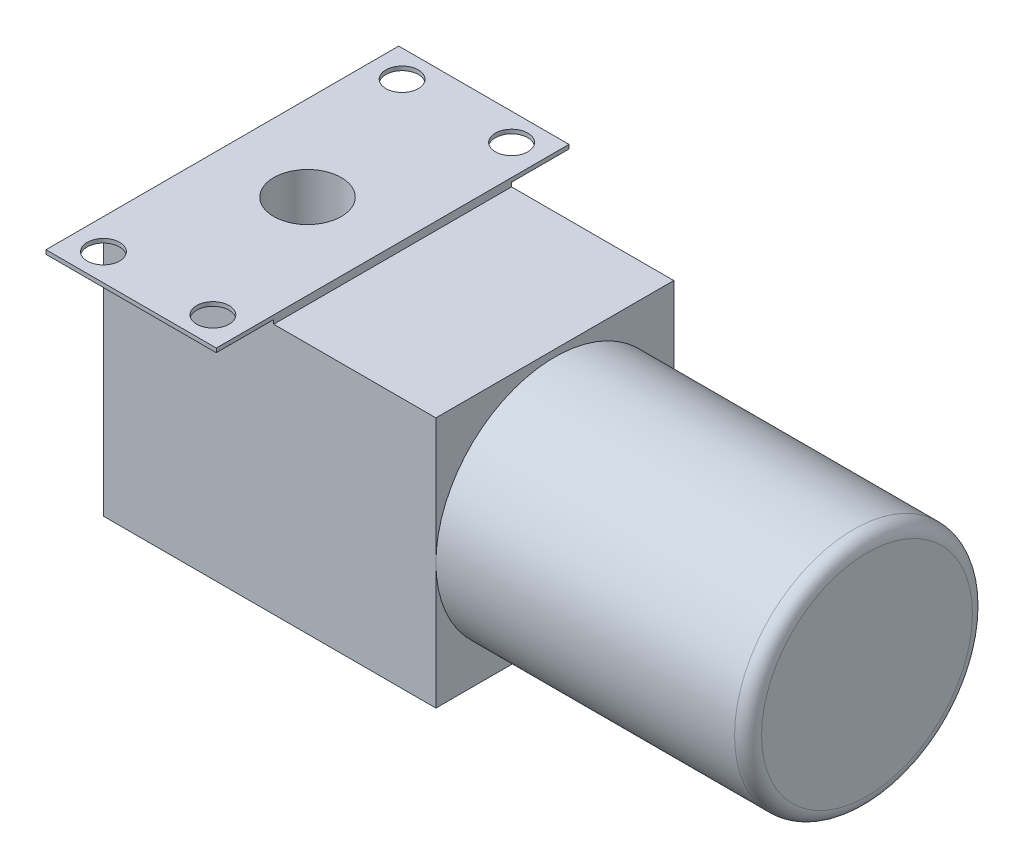
SolidWorks part; units mm, degrees
ref_plane "Front" through (0, 0, 0) normal (0, 0, 1) x (1, 0, 0)
ref_plane "Top" through (0, 0, 0) normal (0, 1, 0) x (1, 0, 0)
ref_plane "Right" through (0, 0, 0) normal (1, 0, 0) x (0, 0, -1)
sketch "草图1" plane through (0, 0, 0) normal (0, 1, 0) x (1, 0, 0)
  line L1 (-31.5, 65.25) -> (31.5, 65.25)
  line L2 (-31.5, 65.25) -> (-31.5, -65.25)
  line L3 (-31.5, -65.25) -> (31.5, -65.25)
  line L4 (31.5, 65.25) -> (31.5, -65.25)
  line L5 (-31.5, 65.25) -> (31.5, -65.25) construction
  line L6 (-31.5, -65.25) -> (31.5, 65.25) construction
  point P0 (0, 0)
  dimension "D1" = 130.5
  dimension "D2" = 63
extrude "凸台-拉伸1" add sketch "草图1" along normal blind 1.5
sketch "草图2" plane through (0, 0, 0) normal (0, -1, 0) x (1, 0, 0)
  line L0 (-31.5, -65.25) -> (-31.5, 65.25) construction
  line L1 (-31.5, 44) -> (91.5, 44)
  line L2 (-31.5, 44) -> (-31.5, -44)
  line L3 (-31.5, -44) -> (91.5, -44)
  line L4 (91.5, 44) -> (91.5, -44)
  line L5 (0, 0) -> (-31.5, 0) construction
  dimension "D1" = 88
  dimension "D2" = 123
extrude "凸台-拉伸2" add sketch "草图2" along normal blind 93 from offset 1.5 separate body
sketch "草图3" plane through (91.5, 0, 0) normal (1, 0, 0) x (0, 0, -1)
  line L0 (-44, -1.5) -> (44, -94.5) construction
  line L1 (44, -94.5) -> (44, -1.5) construction
  circle A0 centre (0, -48) radius 44
extrude "凸台-拉伸3" add sketch "草图3" along normal blind 115.5
sketch "草图5" plane through (0, 0, 0) normal (0, -1, 0) x (1, 0, 0)
  line L0 (-31.5, -44) -> (91.5, -44) construction
  line L1 (-31.5, 44) -> (31.5, 44)
  line L2 (-31.5, 44) -> (-31.5, -44)
  line L3 (-31.5, -44) -> (31.5, -44)
  line L4 (31.5, 44) -> (31.5, -44)
  line L5 (31.5, 65.25) -> (31.5, -65.25) construction
extrude "凸台-拉伸4" add sketch "草图5" along normal blind 3
sketch "草图6" plane through (0, 1.5, 0) normal (0, 1, 0) x (1, 0, 0)
  line L1 (-20.25, 55.25) -> (20.25, 55.25) construction
  line L2 (-20.25, 55.25) -> (-20.25, -55.25) construction
  line L3 (-20.25, -55.25) -> (20.25, -55.25) construction
  line L4 (20.25, 55.25) -> (20.25, -55.25) construction
  line L5 (-20.25, 55.25) -> (20.25, -55.25) construction
  line L6 (-20.25, -55.25) -> (20.25, 55.25) construction
  circle A0 centre (-20.25, 55.25) radius 6
  circle A1 centre (20.25, 55.25) radius 6
  circle A2 centre (-20.25, -55.25) radius 6
  circle A3 centre (20.25, -55.25) radius 6
  point P0 (0, 0)
  dimension "D3" = 12
  dimension "D1" = 40.5
  dimension "D2" = 110.5
extrude "切除-拉伸2" cut sketch "草图6" against normal through all
sketch "草图4" plane through (0, 1.5, 0) normal (0, 1, 0) x (1, 0, 0)
  circle A0 centre (0, 0) radius 12.5
  dimension "D1" = 25
extrude "切除-拉伸1" cut sketch "草图4" against normal through all
fillet "圆角1" radius 5 1 edges at (207, -48, -44)
